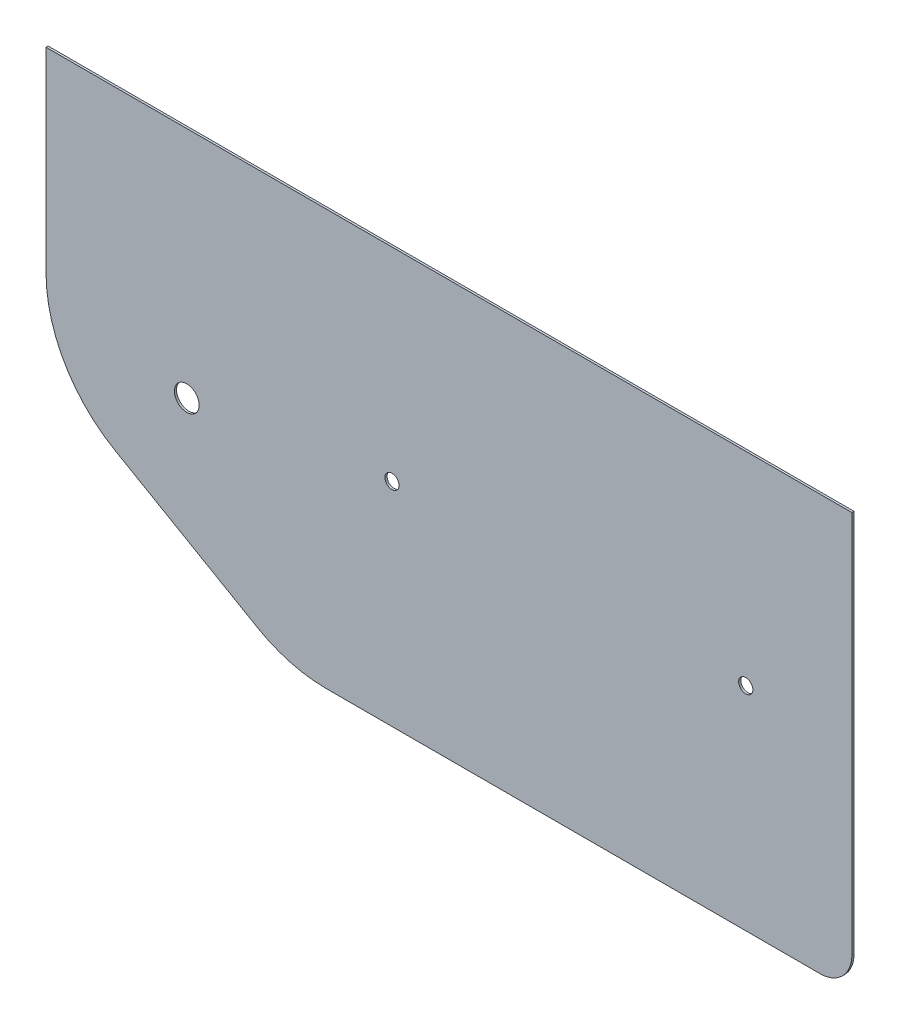
from build123d import *

# Parameters (mm, degrees)
SKETCH1_R           = 10
SKETCH1_R_2         = 17.5
BOSS_EXTRUDE1_DEPTH = 3


with BuildPart() as part:
    # Sketch1 → Boss-Extrude1 (new body)
    with BuildSketch(Plane.XY):
        with BuildLine():
            Line((0, 587), (0, 45))
            ThreePointArc((0, 45), (-13.180194847, 13.180194847), (-45, 0))
            Line((-45, 0), (-742.749907476, 0))
            ThreePointArc((-742.749907476, 0), (-793.219621271, 6.644463874), (-840.249907476, 26.125046262))
            Line((-840.249907476, 26.125046262), (-1041.5, 142.316841355))
            ThreePointArc((-1041.5, 142.316841355), (-1112.874953738, 213.691795093), (-1139, 311.191795093))
            Line((-1139, 311.191795093), (-1139, 587))
            Line((-1139, 587), (0, 587))
        make_face()
        with Locations((-650, 300)):
            Circle(SKETCH1_R, mode=Mode.SUBTRACT)
        with Locations((-150, 300)):
            Circle(SKETCH1_R, mode=Mode.SUBTRACT)
        with Locations((-940, 257)):
            Circle(SKETCH1_R_2, mode=Mode.SUBTRACT)
    extrude(amount=BOSS_EXTRUDE1_DEPTH)


solid = part.part
